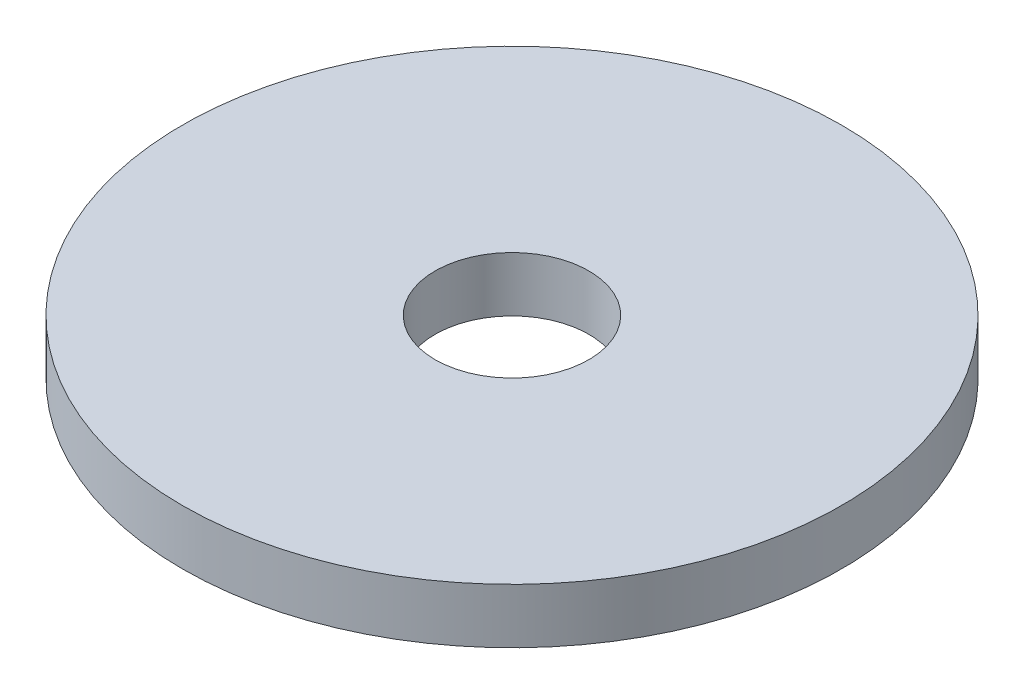
SolidWorks part; units mm, degrees
material "Q235B"
ref_plane "Front Plane" through (0, 0, 0) normal (0, 0, 1) x (1, 0, 0)
ref_plane "Top Plane" through (0, 0, 0) normal (0, 1, 0) x (1, 0, 0)
ref_plane "Right Plane" through (0, 0, 0) normal (1, 0, 0) x (0, 0, -1)
other "Configuration Table"
sketch "Sketch 1" plane through (0, 0, 0) normal (0, 1, 0) x (1, 0, 0)
  circle A1 centre (0, 0) radius 30
  circle A3 centre (0, 0) radius 7
extrude "Boss-Extrude1" add sketch "Sketch 1" along normal blind 5
